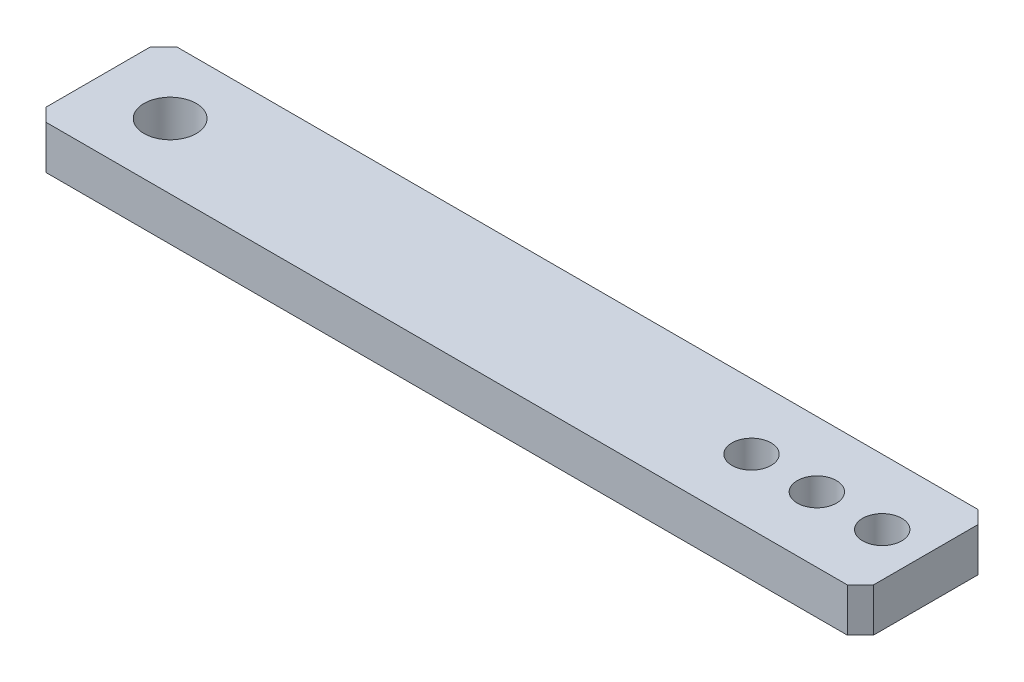
SolidWorks part; units mm, degrees
ref_plane "Front Plane" through (0, 0, 0) normal (0, 0, 1) x (1, 0, 0)
ref_plane "Top Plane" through (0, 0, 0) normal (0, 1, 0) x (1, 0, 0)
ref_plane "Right Plane" through (0, 0, 0) normal (1, 0, 0) x (0, 0, -1)
other "Configuration Table"
sketch "Sketch1" plane through (0, 0, 0) normal (0, 1, 0) x (1, 0, 0)
  line L1 (-95, 15) -> (95, 15)
  line L2 (-95, 15) -> (-95, -15)
  line L3 (-95, -15) -> (95, -15)
  line L4 (95, 15) -> (95, -15)
  line L5 (-95, 15) -> (95, -15) construction
  line L6 (-95, -15) -> (95, 15) construction
  point P0 (0, 0)
  dimension "D1" = 190
  dimension "D2" = 30
extrude "Boss-Extrude1" add sketch "Sketch1" along normal blind 10
chamfer "Chamfer1" distance 3 angle 45 4 edges at (-95, 5, -15) (95, 5, -15) (95, 5, 15) (-95, 5, 15)
hole_wizard "Ø9.0 (9) Diameter Hole1" positions "Sketch2" profile "Sketch3" hole size "Ø9.0" standard "GB"
sketch "Sketch2" plane through (0, 10, 0) normal (0, 1, 0) x (1, 0, 0)
  line L0 (95, -12) -> (95, 12) construction
  point P0 (85, 0)
  point P2 (70, 0)
  point P4 (55, 0)
  dimension "D1" = 10
  dimension "D2" = 15
  dimension "D3" = 30
sketch "Sketch3" plane through (85, 10, 0) normal (1, 0, 0) x (0, 0, 1)
  line L0 (0, 0) -> (0, 22.4539)
  line L1 (0, 22.4539) -> (4.5, 19.75)
  line L2 (4.5, 19.75) -> (4.5, 0)
  line L5 (4.5, 0) -> (0, 0)
  line L10 (0, 22.4539) -> (-4.5, 19.75) construction
  line L11 (0, -6.35) -> (0, 107.95) construction
  dimension "孔直径" = 9
  dimension "孔深度" = 19.75
  dimension "导头角度" = 118
hole_wizard "Ø9.0 (9) Diameter Hole2" positions "Sketch4" profile "Sketch5" hole size "Ø9.0" standard "GB"
sketch "Sketch4" plane through (0, 0, 0) normal (0, -1, 0) x (-1, 0, 0)
  line L0 (95, 12) -> (95, -12) construction
  line L1 (92, -15) -> (-92, -15) construction
  point P5 (78.4924, 0)
  dimension "D1" = 16.5076
  dimension "D2" = 15
sketch "Sketch5" plane through (-78.4924, 0, 0) normal (1, 0, 0) x (0, 0, -1)
  line L0 (0, 0) -> (0, 23.3552)
  line L1 (0, 23.3552) -> (6, 19.75)
  line L2 (6, 19.75) -> (6, 0)
  line L5 (6, 0) -> (0, 0)
  line L10 (0, 23.3552) -> (-6, 19.75) construction
  line L11 (0, -6.35) -> (0, 107.95) construction
  dimension "孔直径" = 12
  dimension "孔深度" = 19.75
  dimension "导头角度" = 118
